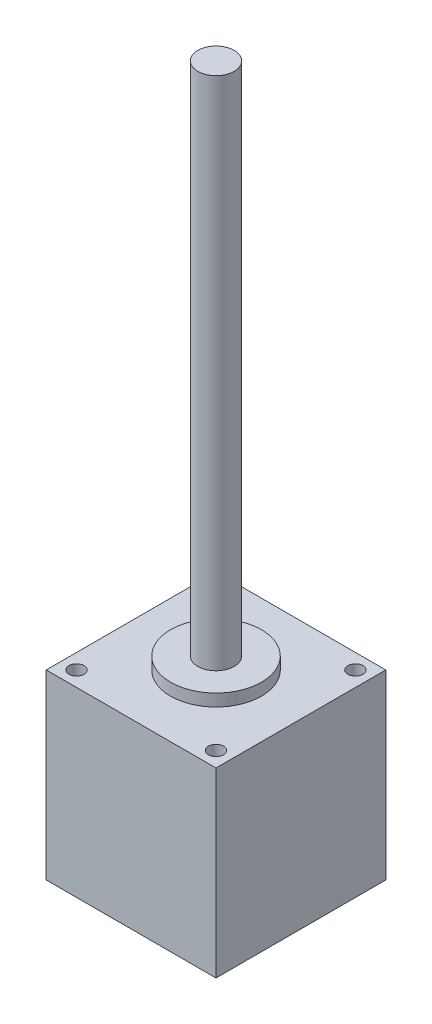
SolidWorks part; units mm, degrees
material "20#"
ref_plane "Front Plane" through (0, 0, 0) normal (0, 0, 1) x (1, 0, 0)
ref_plane "Top Plane" through (0, 0, 0) normal (0, 1, 0) x (1, 0, 0)
ref_plane "Right Plane" through (0, 0, 0) normal (1, 0, 0) x (0, 0, -1)
sketch "Sketch1" plane through (0, 0, 0) normal (0, 1, 0) x (1, 0, 0)
  line L1 (-14, 14) -> (14, 14)
  line L2 (-14, 14) -> (-14, -14)
  line L3 (-14, -14) -> (14, -14)
  line L4 (14, 14) -> (14, -14)
  line L5 (-14, 14) -> (14, -14) construction
  line L6 (-14, -14) -> (14, 14) construction
  point P0 (0, 0)
  dimension "D1" = 28
extrude "Boss-Extrude1" add sketch "Sketch1" along normal blind 30
sketch "Sketch2" plane through (0, 30, 0) normal (0, 1, 0) x (1, 0, 0)
  circle A0 centre (0, 0) radius 7.5
  dimension "D1" = 15
extrude "Boss-Extrude2" add sketch "Sketch2" along normal blind 2
sketch "Sketch3" plane through (0, 32, 0) normal (0, 1, 0) x (1, 0, 0)
  circle A0 centre (0, 0) radius 3
  dimension "D1" = 6
extrude "Boss-Extrude3" add sketch "Sketch3" along normal blind 85
cosmetic thread "Cosmetic Thread1" parameters "D2"=4.917
sketch "Sketch4" plane through (0, 30, 0) normal (0, 1, 0) x (1, 0, 0)
  line L1 (-11.5, 11.5) -> (11.5, 11.5) construction
  line L2 (-11.5, 11.5) -> (-11.5, -11.5) construction
  line L3 (-11.5, -11.5) -> (11.5, -11.5) construction
  line L4 (11.5, 11.5) -> (11.5, -11.5) construction
  line L5 (-11.5, 11.5) -> (11.5, -11.5) construction
  line L6 (-11.5, -11.5) -> (11.5, 11.5) construction
  circle A2 centre (-11.5, -11.5) radius 1
  circle A3 centre (11.5, -11.5) radius 1
  circle A4 centre (-11.5, 11.5) radius 1
  circle A5 centre (11.5, 11.5) radius 1
  point P0 (0, 0)
  dimension "D4" = 2
  dimension "D1" = 23
  dimension "D2" = 23
extrude "Cut-Extrude1" cut sketch "Sketch4" against normal blind 3
hole_wizard "M3 Tapped Hole1" positions "Sketch7" profile "Sketch8" tap size "M3" standard "GB"
sketch "Sketch7" plane through (0, 30, 0) normal (0, 1, 0) x (1, 0, 0)
  point P0 (-11.5, -11.5)
  point P3 (11.5, -11.5)
  point P6 (-11.5, 11.5)
  point P8 (11.5, 11.5)
sketch "Sketch8" plane through (-11.5, 30, 11.5) normal (1, 0, 0) x (0, 0, 1)
  line L0 (0, 0) -> (0, 8.2511)
  line L1 (0, 8.2511) -> (1.25, 7.5)
  line L2 (1.25, 7.5) -> (1.25, 0)
  line L5 (1.25, 0) -> (0, 0)
  line L10 (0, 8.2511) -> (-1.25, 7.5) construction
  line L11 (0, -6.35) -> (0, 107.95) construction
  dimension "螺纹孔钻头直径" = 2.5
  dimension "螺纹孔钻头深度" = 7.5
  dimension "导头角度" = 118
cosmetic thread "HoleThreadLine3" parameters "D1"=6, "D2"=3
cosmetic thread "HoleThreadLine4" parameters "D1"=6, "D2"=3
cosmetic thread "HoleThreadLine5" parameters "D1"=6, "D2"=3
cosmetic thread "HoleThreadLine6" parameters "D1"=6, "D2"=3
